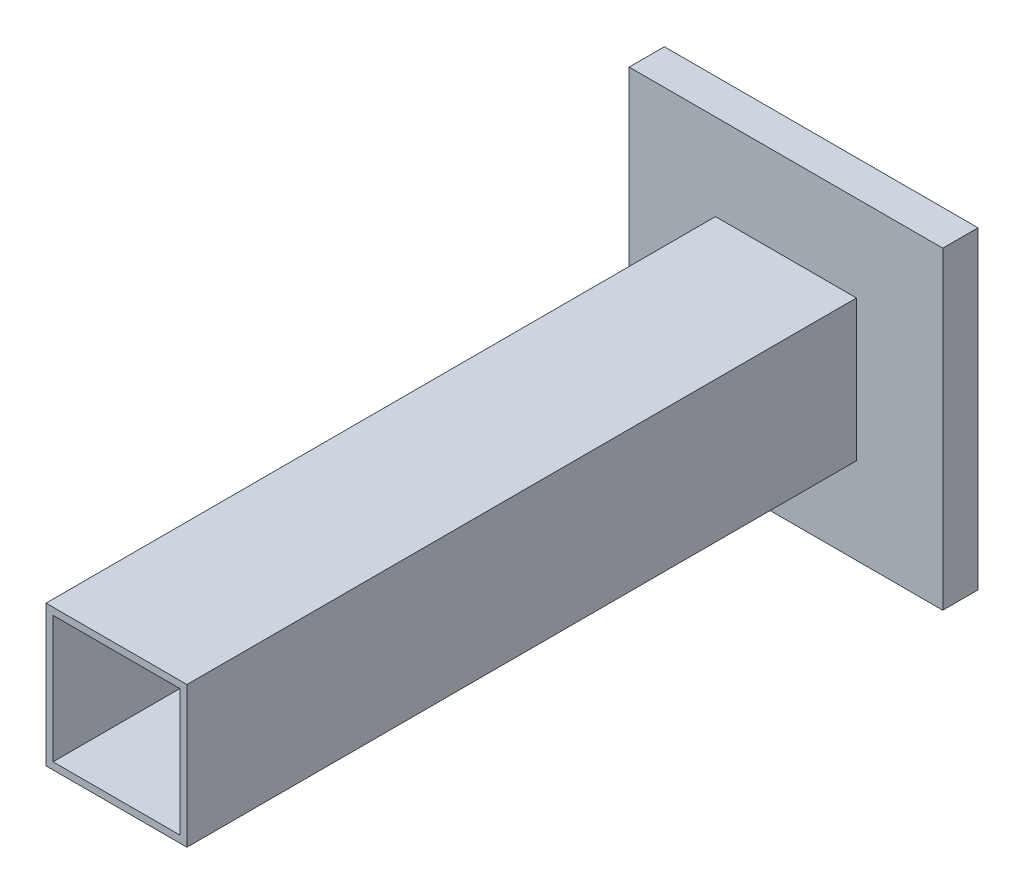
from build123d import *

# Parameters (mm, degrees)
SKETCH1_W           = 445
SKETCH1_H           = 445
BOSS_EXTRUDE1_DEPTH = 50
SKETCH2_W           = 200
SKETCH2_H           = 200
SKETCH2_W_2         = 180
SKETCH2_H_2         = 180
BOSS_EXTRUDE2_DEPTH = 950


with BuildPart() as part:
    # Sketch1 → Boss-Extrude1 (new body)
    with BuildSketch(Plane.XY):
        Rectangle(SKETCH1_W, SKETCH1_H)
    extrude(amount=BOSS_EXTRUDE1_DEPTH)

    # Sketch2 → Boss-Extrude2 (add)
    with BuildSketch(Plane.XY.offset(50)):
        Rectangle(SKETCH2_W, SKETCH2_H)
        Rectangle(SKETCH2_W_2, SKETCH2_H_2, mode=Mode.SUBTRACT)
    extrude(amount=BOSS_EXTRUDE2_DEPTH)


solid = part.part
